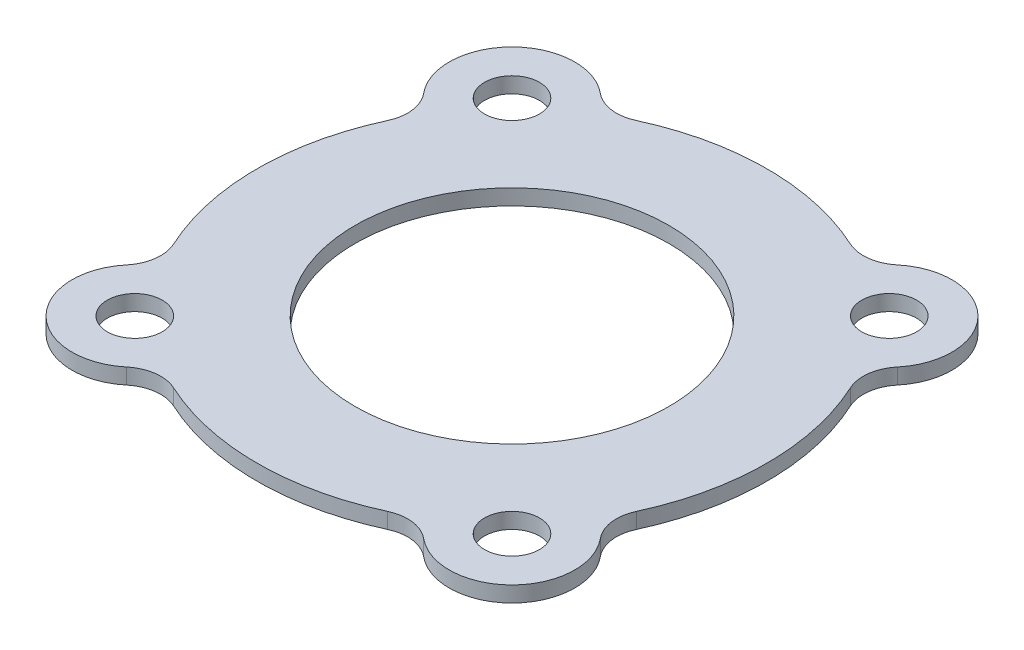
from build123d import *

# Parameters (mm, degrees)
SKETCH2_R           = 20
SKETCH2_R_2         = 3.5
BOSS_EXTRUDE1_DEPTH = 2
FILLET1_R           = 5
FILLET2_R           = 5


with BuildPart() as part:
    # Sketch2 → Boss-Extrude1 (new body)
    with BuildSketch(Plane(origin=(0, 0, 0), x_dir=(1, 0, 0), z_dir=(0, 1, 0))):
        with BuildLine():
            ThreePointArc((-27.733348113, 16.944361965), (-32.5, 0), (-27.733348113, -16.944361965))
            ThreePointArc((-27.733348113, -16.944361965), (-29.69848481, -29.69848481), (-16.944361965, -27.733348113))
            ThreePointArc((-16.944361965, -27.733348113), (0, -32.5), (16.944361965, -27.733348113))
            ThreePointArc((16.944361965, -27.733348113), (29.69848481, -29.69848481), (27.733348113, -16.944361965))
            ThreePointArc((27.733348113, -16.944361965), (32.5, 0), (27.733348113, 16.944361965))
            ThreePointArc((27.733348113, 16.944361965), (29.69848481, 29.69848481), (16.944361965, 27.733348113))
            ThreePointArc((16.944361965, 27.733348113), (0, 32.5), (-16.944361965, 27.733348113))
            ThreePointArc((-16.944361965, 27.733348113), (-29.69848481, 29.69848481), (-27.733348113, 16.944361965))
        make_face()
        with Locations(Location((0, 0, 0), (0, 0, 270))):
            Circle(SKETCH2_R, mode=Mode.SUBTRACT)
        with Locations(Location((-24.04163056, 24.04163056, 0), (0, 0, 270))):
            Circle(SKETCH2_R_2, mode=Mode.SUBTRACT)
        with Locations(Location((24.04163056, 24.04163056, 0), (0, 0, 270))):
            Circle(SKETCH2_R_2, mode=Mode.SUBTRACT)
        with Locations(Location((24.04163056, -24.04163056, 0), (0, 0, 270))):
            Circle(SKETCH2_R_2, mode=Mode.SUBTRACT)
        with Locations(Location((-24.04163056, -24.04163056, 0), (0, 0, 270))):
            Circle(SKETCH2_R_2, mode=Mode.SUBTRACT)
    extrude(amount=BOSS_EXTRUDE1_DEPTH)

    # Fillet1
    fillet1_edges = [part.edges().sort_by_distance(p)[0] for p in [
        (16.944361965, 1, -27.733348113),
        (27.733348113, 1, -16.944361965),
        (27.733348113, 1, 16.944361965),
        (16.944361965, 1, 27.733348113),
        (-16.944361965, 1, 27.733348113),
        (-27.733348113, 1, 16.944361965),
        (-27.733348113, 1, -16.944361965),
    ]]
    fillet(fillet1_edges, radius=FILLET1_R)

    # Fillet2
    fillet2_edges = [part.edges().sort_by_distance(p)[0] for p in [
        (-16.944361965, 1, -27.733348113),
    ]]
    fillet(fillet2_edges, radius=FILLET2_R)


solid = part.part
